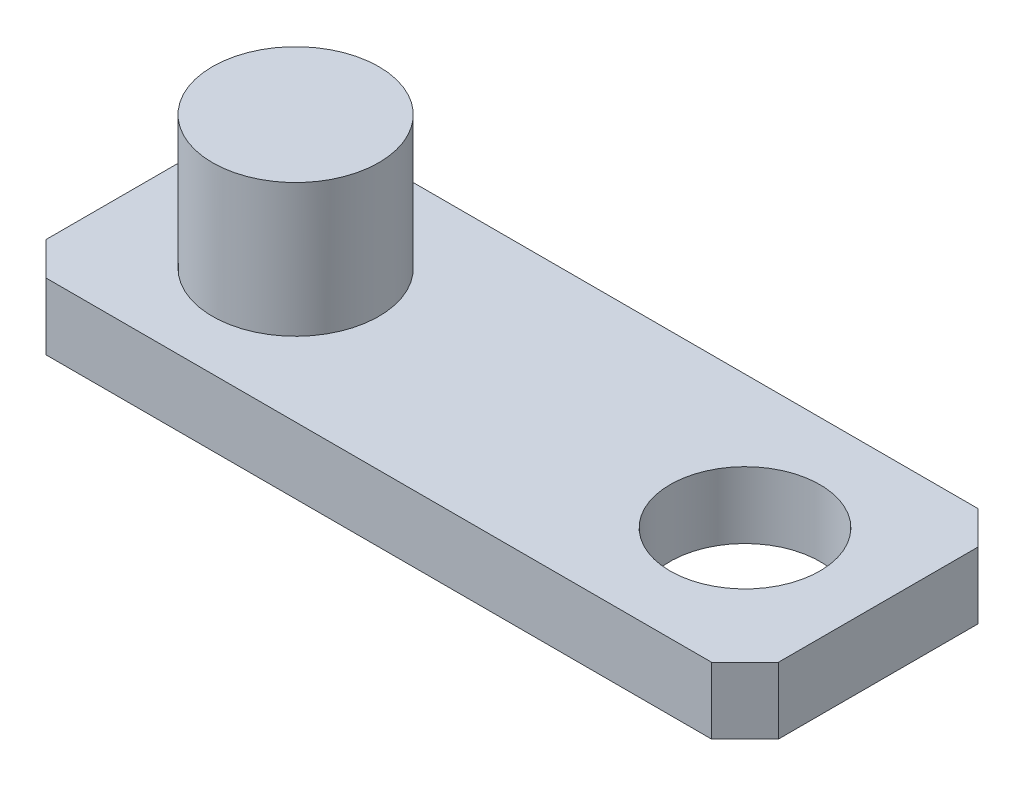
SolidWorks part; units mm, degrees
ref_plane "Front Plane" through (0, 0, 0) normal (0, 0, 1) x (1, 0, 0)
ref_plane "Top Plane" through (0, 0, 0) normal (0, 1, 0) x (1, 0, 0)
ref_plane "Right Plane" through (0, 0, 0) normal (1, 0, 0) x (0, 0, -1)
sketch "Sketch1" plane through (0, 0, 0) normal (0, 1, 0) x (1, 0, 0)
  line L1 (-11, -4) -> (11, -4)
  line L2 (-11, -4) -> (-11, 4)
  line L3 (-11, 4) -> (11, 4)
  line L4 (11, -4) -> (11, 4)
  line L5 (-11, -4) -> (11, 4) construction
  line L6 (-11, 4) -> (11, -4) construction
  point P0 (0, 0)
  dimension "D1" = 8
  dimension "D2" = 22
extrude "Boss-Extrude1" add sketch "Sketch1" along normal blind 2
sketch "Sketch2" plane through (0, 2, 0) normal (0, 1, 0) x (1, 0, 0)
  line L0 (11, -4) -> (11, 4) construction
  circle A0 centre (7, 0) radius 2.25
  dimension "D1" = 4.5
  dimension "D2" = 4
extrude "Cut-Extrude1" cut sketch "Sketch2" against normal through all
sketch "Sketch3" plane through (0, 2, 0) normal (0, 1, 0) x (1, 0, 0)
  circle A0 centre (-6.5, 0) radius 2.5
  circle A1 centre (7, 0) radius 2.25 construction
  dimension "D1" = 5
  dimension "D2" = 13.5
extrude "Boss-Extrude2" add sketch "Sketch3" along normal blind 4
chamfer "Chamfer1" distance 1 angle 45 4 edges at (11, 1, -4) (11, 1, 4) (-11, 1, -4) (-11, 1, 4)
